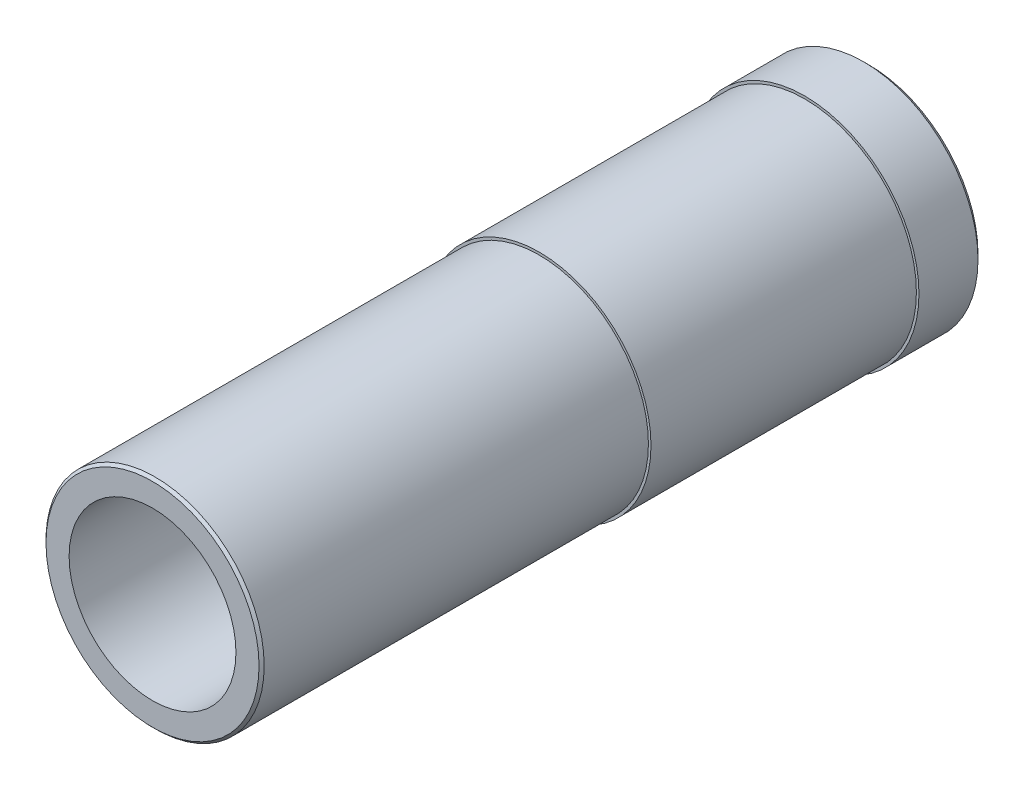
from build123d import *

# Parameters (mm, degrees)
SKETCH_1_R          = 44.5
SKETCH_1_R_2        = 32.5
EXTRUDE_1_DEPTH     = 279.1
SKETCH_2_R          = 44.5
SKETCH_2_R_2        = 43.5
CUT_EXTRUDE_1_DEPTH = 254.1
CUT_EXTRUDE_START   = -150.7
SKETCH_3_R          = 43.5
SKETCH_3_R_2        = 42.5
CUT_EXTRUDE_2_DEPTH = 150.7
CHAMFER_1_SIZE      = 2
CHAMFER_2_SIZE      = 1


with BuildPart() as part:
    # 草图1 → 凸台-拉伸1 (new body)
    with BuildSketch(Plane.XY):
        Circle(SKETCH_1_R)
        Circle(SKETCH_1_R_2, mode=Mode.SUBTRACT)
    extrude(amount=EXTRUDE_1_DEPTH)

    # 草图2 → 切除-拉伸1 (cut)
    with BuildSketch(Plane(origin=(0, 0, 25), x_dir=(-1, 0, 0), z_dir=(0, 0, -1))):
        Circle(SKETCH_2_R)
        Circle(SKETCH_2_R_2, mode=Mode.SUBTRACT)
    extrude(amount=-CUT_EXTRUDE_1_DEPTH, mode=Mode.SUBTRACT)

    # 草图3 → 切除-拉伸2 (cut)
    with BuildSketch(Plane.XY.offset(279.1).offset(CUT_EXTRUDE_START)):
        with Locations(Location((0, 0, 0), (0, 0, 180))):
            Circle(SKETCH_3_R)
        Circle(SKETCH_3_R_2, mode=Mode.SUBTRACT)
    extrude(amount=CUT_EXTRUDE_2_DEPTH, mode=Mode.SUBTRACT)

    # 倒角1
    chamfer_1_edges = [part.edges().sort_by_distance(p)[0] for p in [
        (-44.5, 0, 0),
    ]]
    chamfer(chamfer_1_edges, length=CHAMFER_1_SIZE)

    # 倒角2
    chamfer_2_edges = [part.edges().sort_by_distance(p)[0] for p in [
        (-42.5, 0, 279.1),
    ]]
    chamfer(chamfer_2_edges, length=CHAMFER_2_SIZE)


solid = part.part
